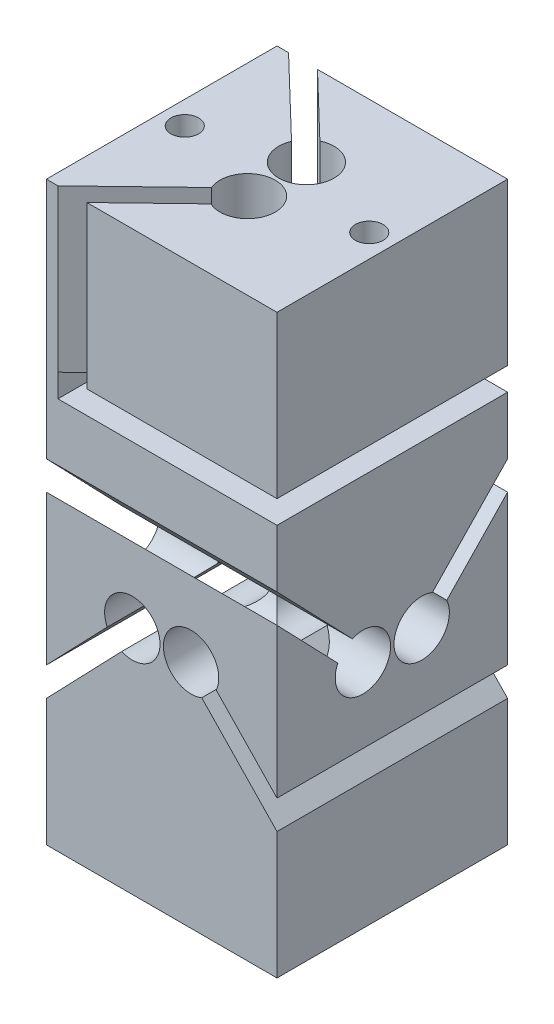
SolidWorks part; units mm, degrees
ref_plane "Front Plane" through (0, 0, 0) normal (0, 0, 1) x (1, 0, 0)
ref_plane "Top Plane" through (0, 0, 0) normal (0, 1, 0) x (1, 0, 0)
ref_plane "Right Plane" through (0, 0, 0) normal (1, 0, 0) x (0, 0, -1)
sketch "Sketch1" plane through (0, 0, 0) normal (0, 1, 0) x (1, 0, 0)
  line L1 (-5, -5) -> (5, -5)
  line L2 (-5, -5) -> (-5, 5)
  line L3 (-5, 5) -> (5, 5)
  line L4 (5, -5) -> (5, 5)
  line L5 (-5, -5) -> (5, 5) construction
  line L6 (-5, 5) -> (5, -5) construction
  point P0 (0, 0)
  dimension "D1" = 10
  dimension "D2" = 10
extrude "Boss-Extrude1" add sketch "Sketch1" along normal blind 10
sketch "Sketch2" plane through (0, 0, 5) normal (0, 0, 1) x (1, 0, 0)
  line L0 (-5, 0) -> (5, 0) construction
  line L1 (2.3638, 4.4955) -> (5, 1.755)
  line L2 (1.7368, 3.8924) -> (5, 0.5)
  line L4 (5, 1.755) -> (5, 0.5)
  line L5 (5, 10) -> (5, 0) construction
  line L6 (0, -1000) -> (0, 49000) construction
  line L7 (-5, 1.755) -> (-5, 0.5)
  line L8 (-1.7368, 3.8924) -> (-5, 0.5)
  line L9 (-2.3638, 4.4955) -> (-5, 1.755)
  arc A0 (-1.7368, 3.8924) -> (-2.3638, 4.4955) centre (-1.275, 5) ccw
  arc A1 (2.3638, 4.4955) -> (1.7368, 3.8924) centre (1.275, 5) ccw
  point P15 (0, 0)
  dimension "D1" = 2.4
  dimension "D3" = 0.87
  dimension "D4" = 5
  dimension "D5" = 1.275
  dimension "D7" = 0.5
  dimension "D6" = 0.435
extrude "Cut-Extrude1" cut sketch "Sketch2" against normal through all
sketch "Sketch3" plane through (5, 0, 0) normal (1, 0, 0) x (0, 0, -1)
  line L26 (-5, 8.245) -> (-5, 9.5)
  line L27 (5, 8.245) -> (5, 9.5)
  line L28 (1.7368, 6.1076) -> (5, 9.5)
  line L29 (2.3638, 5.5045) -> (5, 8.245)
  line L30 (5, 8.245) -> (5, 9.5)
  line L31 (1.7368, 6.1076) -> (5, 9.5)
  line L32 (2.3638, 5.5045) -> (5, 8.245)
  line L33 (5, 8.245) -> (5, 9.5)
  line L34 (1.7368, 6.1076) -> (5, 9.5)
  line L35 (2.3638, 5.5045) -> (5, 8.245)
  line L36 (5, 8.245) -> (5, 9.5)
  line L37 (1.7368, 6.1076) -> (5, 9.5)
  line L38 (2.3638, 5.5045) -> (5, 8.245)
  line L39 (-2.3638, 5.5045) -> (-5, 8.245)
  line L40 (-1.7368, 6.1076) -> (-5, 9.5)
  line L41 (-2.3638, 5.5045) -> (-5, 8.245)
  line L42 (-1.7368, 6.1076) -> (-5, 9.5)
  line L43 (-2.3638, 5.5045) -> (-5, 8.245)
  line L44 (-1.7368, 6.1076) -> (-5, 9.5)
  line L45 (-2.3638, 5.5045) -> (-5, 8.245)
  line L46 (-1.7368, 6.1076) -> (-5, 9.5)
  arc A8 (1.7368, 6.1076) -> (2.3638, 5.5045) centre (1.275, 5) ccw
  arc A9 (2.3638, 5.5045) -> (1.7368, 6.1076) centre (1.275, 5) cw
  arc A10 (1.7368, 6.1076) -> (2.3638, 5.5045) centre (1.275, 5) ccw
  arc A11 (2.3638, 5.5045) -> (1.7368, 6.1076) centre (1.275, 5) cw
  arc A12 (-2.3638, 5.5045) -> (-1.7368, 6.1076) centre (-1.275, 5) ccw
  arc A13 (-1.7368, 6.1076) -> (-2.3638, 5.5045) centre (-1.275, 5) cw
  arc A14 (-2.3638, 5.5045) -> (-1.7368, 6.1076) centre (-1.275, 5) ccw
  arc A15 (-1.7368, 6.1076) -> (-2.3638, 5.5045) centre (-1.275, 5) cw
  line M3 (-5, 10) -> (-5, 1.755)
  line M5 (5, 1.755) -> (5, 10)
  dimension "D1" = 0.5
  dimension "D2" = 0.5
extrude "Cut-Extrude2" cut sketch "Sketch3" against normal through all contours L28 A8 L29 M5 | L39 A12 L40 M3
sketch "Sketch4" plane through (0, 0, 0) normal (0, -1, 0) x (1, 0, 0)
  line L4 (5, -5) -> (5, 5)
  line L5 (5, 5) -> (-5, 5)
  line L6 (-5, 5) -> (-5, -5)
  line L7 (-5, -5) -> (5, -5)
  line L8 (5, -5) -> (5, 5)
  line L9 (5, 5) -> (-5, 5)
  line L10 (-5, 5) -> (-5, -5)
  line L11 (-5, -5) -> (5, -5)
  dimension "D1" = 0
extrude "Boss-Extrude2" add sketch "Sketch4" along normal blind 5
sketch "Sketch5" plane through (0, 10, 0) normal (0, 1, 0) x (1, 0, 0)
  line L4 (5, -5) -> (5, 5)
  line L5 (5, 5) -> (-5, 5)
  line L6 (-5, 5) -> (-5, -5)
  line L7 (-5, -5) -> (5, -5)
  line L8 (5, -5) -> (5, 5)
  line L9 (5, 5) -> (-5, 5)
  line L10 (-5, 5) -> (-5, -5)
  line L11 (-5, -5) -> (5, -5)
  dimension "D1" = 0
extrude "Boss-Extrude3" add sketch "Sketch5" along normal blind 10
sketch "Sketch7" plane through (0, 20, 0) normal (0, 1, 0) x (1, 0, 0)
  line L0 (-0.5045, -2.3638) -> (-3.245, -5)
  line L1 (-1.1076, -1.7368) -> (-4.5, -5)
  line L2 (-3.245, -5) -> (-4.5, -5)
  line L3 (-3.245, 5) -> (-4.5, 5)
  line L4 (-1.1076, 1.7368) -> (-4.5, 5)
  line L5 (-0.5045, 2.3638) -> (-3.245, 5)
  arc A0 (-1.1076, 1.7368) -> (-0.5045, 2.3638) centre (0, 1.275) ccw
  arc A1 (-0.5045, -2.3638) -> (-1.1076, -1.7368) centre (0, -1.275) ccw
  dimension "D1" = 0.87
  dimension "D2" = 0.435
  dimension "D3" = 0.5
  dimension "D4" = 0.5
extrude "Cut-Extrude3" cut sketch "Sketch7" against normal blind 8
sketch "Sketch8" plane through (5, 0, 0) normal (1, 0, 0) x (0, 0, -1)
  line L0 (-5, 20) -> (-5, 9.5) construction
  line L1 (-5, 13) -> (5, 13)
  line L2 (-5, 13) -> (-5, 12)
  line L3 (-5, 12) -> (5, 12)
  line L4 (5, 13) -> (5, 12)
  line L5 (5, 20) -> (5, 9.5) construction
  line L6 (-5, 20) -> (5, 20) construction
  dimension "D1" = 1
  dimension "D2" = 8
extrude "Cut-Extrude4" cut sketch "Sketch8" against normal up to vertex (9.5 mm away)
sketch "Sketch9" plane through (0, 20, 0) normal (0, 1, 0) x (1, 0, 0)
  circle A0 centre (0, 0) radius 3.8382
sketch "Sketch10" plane through (0, -5, 0) normal (0, -1, 0) x (1, 0, 0)
  line L0 (0, 0) -> (0, 4) construction
  line L1 (0, 0) -> (-2.8284, 2.8284) construction
  circle A0 centre (0, 0) radius 4 construction
  circle A2 centre (-2.8284, 2.8284) radius 1
  circle A3 centre (2.8284, 2.8284) radius 1
  circle A4 centre (2.8284, -2.8284) radius 1
  circle A5 centre (-2.8284, -2.8284) radius 1
  point P15 (0, 0)
  dimension "D1" = 8
  dimension "D2" = 45
  dimension "D3" = 2
  dimension "D4" = 4
extrude "Cut-Extrude5" cut sketch "Sketch10" against normal blind 5
sketch "Sketch11" plane through (0, 20, 0) normal (0, 1, 0) x (1, 0, 0)
  circle A0 centre (0, 0) radius 4 construction
  circle A1 centre (4, 0) radius 0.6
  circle A2 centre (-4, 0) radius 0.6
  dimension "D1" = 8
  dimension "D2" = 1.2
  dimension "D3" = 1.2
extrude "Cut-Extrude6" cut sketch "Sketch11" against normal blind 5
